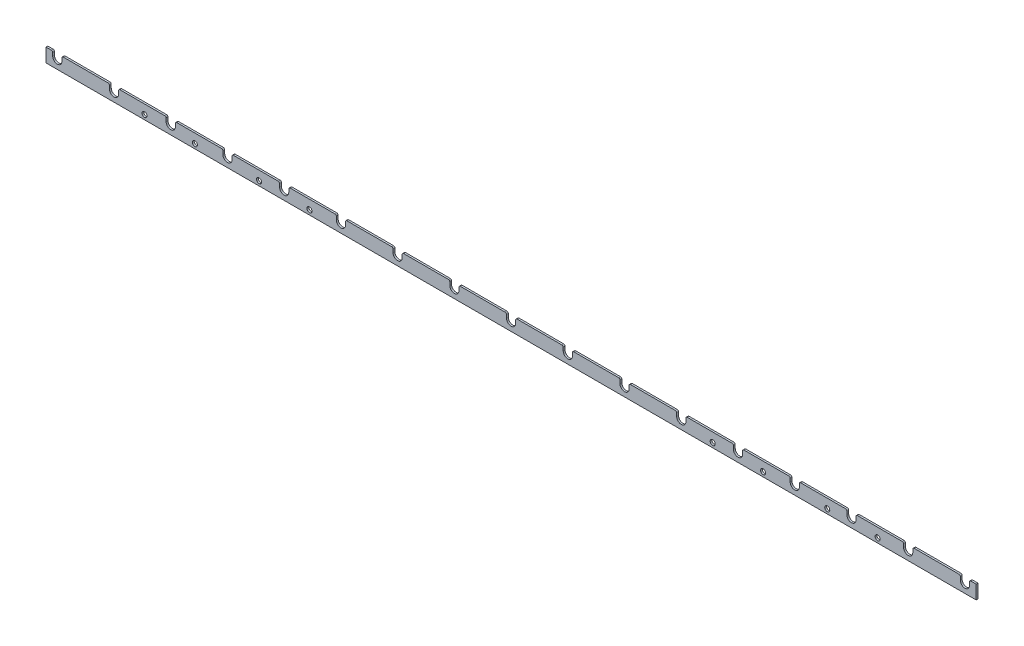
SolidWorks part; units mm, degrees
ref_plane "前视基准面" through (0, 0, 0) normal (0, 0, 1) x (1, 0, 0)
ref_plane "上视基准面" through (0, 0, 0) normal (0, 1, 0) x (1, 0, 0)
ref_plane "右视基准面" through (0, 0, 0) normal (1, 0, 0) x (0, 0, -1)
sketch "草图1" plane through (0, 0, 0) normal (0, 0, 1) x (1, 0, 0)
  line L1 (1015, 15) -> (-1015, 15)
  line L2 (1015, 15) -> (1015, -15)
  line L3 (1015, -15) -> (-1015, -15)
  line L4 (-1015, 15) -> (-1015, -15)
  line L5 (1015, 15) -> (-1015, -15) construction
  line L6 (1015, -15) -> (-1015, 15) construction
  point P0 (0, 0)
  dimension "D1" = 2030
  dimension "D2" = 30
extrude "凸台-拉伸1" add sketch "草图1" along normal blind 4
sketch "草图2" plane through (0, 0, 4) normal (0, 0, 1) x (1, 0, 0)
  line L0 (1015, 15) -> (-1015, 15) construction
  line L1 (-1000.4, 5) -> (-980.4, 5) construction
  line L2 (-1015, 15) -> (-1015, -15) construction
  line L3 (-1000.4, 5) -> (-1000.4, 15)
  line L4 (-980.4, 5) -> (-980.4, 15)
  line L5 (-980.4, 15) -> (-1000.4, 15)
  line L6 (-856.6, 15) -> (-876.6, 15)
  line L7 (-876.6, 5) -> (-876.6, 15)
  line L8 (-856.6, 5) -> (-856.6, 15)
  line L9 (-732.8, 15) -> (-752.8, 15)
  line L10 (-752.8, 5) -> (-752.8, 15)
  line L11 (-732.8, 5) -> (-732.8, 15)
  line L12 (-609, 15) -> (-629, 15)
  line L13 (-629, 5) -> (-629, 15)
  line L14 (-609, 5) -> (-609, 15)
  line L15 (-485.2, 15) -> (-505.2, 15)
  line L16 (-505.2, 5) -> (-505.2, 15)
  line L17 (-485.2, 5) -> (-485.2, 15)
  line L18 (-361.4, 15) -> (-381.4, 15)
  line L19 (-381.4, 5) -> (-381.4, 15)
  line L20 (-361.4, 5) -> (-361.4, 15)
  line L21 (-237.6, 15) -> (-257.6, 15)
  line L22 (-257.6, 5) -> (-257.6, 15)
  line L23 (-237.6, 5) -> (-237.6, 15)
  line L24 (-113.8, 15) -> (-133.8, 15)
  line L25 (-133.8, 5) -> (-133.8, 15)
  line L26 (-113.8, 5) -> (-113.8, 15)
  line L27 (10, 15) -> (-10, 15)
  line L28 (-10, 5) -> (-10, 15)
  line L29 (10, 5) -> (10, 15)
  line L30 (133.8, 15) -> (113.8, 15)
  line L31 (113.8, 5) -> (113.8, 15)
  line L32 (133.8, 5) -> (133.8, 15)
  line L33 (257.6, 15) -> (237.6, 15)
  line L34 (237.6, 5) -> (237.6, 15)
  line L35 (257.6, 5) -> (257.6, 15)
  line L36 (381.4, 15) -> (361.4, 15)
  line L37 (361.4, 5) -> (361.4, 15)
  line L38 (381.4, 5) -> (381.4, 15)
  line L39 (505.2, 15) -> (485.2, 15)
  line L40 (485.2, 5) -> (485.2, 15)
  line L41 (505.2, 5) -> (505.2, 15)
  line L42 (629, 15) -> (609, 15)
  line L43 (609, 5) -> (609, 15)
  line L44 (629, 5) -> (629, 15)
  line L45 (752.8, 15) -> (732.8, 15)
  line L46 (732.8, 5) -> (732.8, 15)
  line L47 (752.8, 5) -> (752.8, 15)
  line L48 (876.6, 15) -> (856.6, 15)
  line L49 (856.6, 5) -> (856.6, 15)
  line L50 (876.6, 5) -> (876.6, 15)
  line L51 (1000.4, 15) -> (980.4, 15)
  line L52 (980.4, 5) -> (980.4, 15)
  line L53 (1000.4, 5) -> (1000.4, 15)
  arc A0 (-996.9, 5) -> (-983.9, 5) centre (-990.4, 5) ccw construction
  arc A1 (-1000.4, 5) -> (-980.4, 5) centre (-990.4, 5) ccw
  arc A2 (-876.6, 5) -> (-856.6, 5) centre (-866.6, 5) ccw
  arc A3 (-752.8, 5) -> (-732.8, 5) centre (-742.8, 5) ccw
  arc A4 (-629, 5) -> (-609, 5) centre (-619, 5) ccw
  arc A5 (-505.2, 5) -> (-485.2, 5) centre (-495.2, 5) ccw
  arc A6 (-381.4, 5) -> (-361.4, 5) centre (-371.4, 5) ccw
  arc A7 (-257.6, 5) -> (-237.6, 5) centre (-247.6, 5) ccw
  arc A8 (-133.8, 5) -> (-113.8, 5) centre (-123.8, 5) ccw
  arc A9 (-10, 5) -> (10, 5) centre (0, 5) ccw
  arc A10 (113.8, 5) -> (133.8, 5) centre (123.8, 5) ccw
  arc A11 (237.6, 5) -> (257.6, 5) centre (247.6, 5) ccw
  arc A12 (361.4, 5) -> (381.4, 5) centre (371.4, 5) ccw
  arc A13 (485.2, 5) -> (505.2, 5) centre (495.2, 5) ccw
  arc A14 (609, 5) -> (629, 5) centre (619, 5) ccw
  arc A15 (732.8, 5) -> (752.8, 5) centre (742.8, 5) ccw
  arc A16 (856.6, 5) -> (876.6, 5) centre (866.6, 5) ccw
  arc A17 (980.4, 5) -> (1000.4, 5) centre (990.4, 5) ccw
  dimension "D2" = 13
  dimension "D3" = 20
  dimension "D4" = 24.6
  dimension "D1" = 10
  dimension "D5" = 17
extrude "切除-拉伸1" cut sketch "草图2" against normal blind 4
fillet "圆角1" radius 3 34 edges at (980.4, 15, 2) (1000.4, 15, 2) (856.6, 15, 2) (876.6, 15, 2) (732.8, 15, 2) (752.8, 15, 2) (609, 15, 2) (629, 15, 2) (485.2, 15, 2) (505.2, 15, 2) (361.4, 15, 2) (381.4, 15, 2) (237.6, 15, 2) (257.6, 15, 2) (113.8, 15, 2) (133.8, 15, 2) (-10, 15, 2) (10, 15, 2) (-133.8, 15, 2) (-113.8, 15, 2) (-257.6, 15, 2) (-237.6, 15, 2) (-381.4, 15, 2) (-361.4, 15, 2) (-505.2, 15, 2) (-485.2, 15, 2) (-629, 15, 2) (-609, 15, 2) (-752.8, 15, 2) (-732.8, 15, 2) (-876.6, 15, 2) (-856.6, 15, 2) (-1000.4, 15, 2) (-980.4, 15, 2)
sketch "草图3" plane through (0, 0, 4) normal (0, 0, 1) x (1, 0, 0)
  line L1 (0, 0) -> (0, 125.9014) construction
  circle A0 centre (-800, -5) radius 5.5
  circle A1 centre (-690, -5) radius 5.5
  circle A2 centre (-550, -5) radius 5.5
  circle A3 centre (-440, -5) radius 5.5
  arc A4 (-752.8, 5) -> (-732.8, 5) centre (-742.8, 5) ccw construction
  circle A5 centre (440, -5) radius 5.5
  circle A6 centre (550, -5) radius 5.5
  circle A7 centre (690, -5) radius 5.5
  circle A8 centre (800, -5) radius 5.5
  dimension "D2" = 140
  dimension "D3" = 110
  dimension "D4" = 440
  dimension "D5" = 11
  dimension "D6" = 10
  dimension "D1" = 110
extrude "切除-拉伸2" cut sketch "草图3" against normal blind 4
